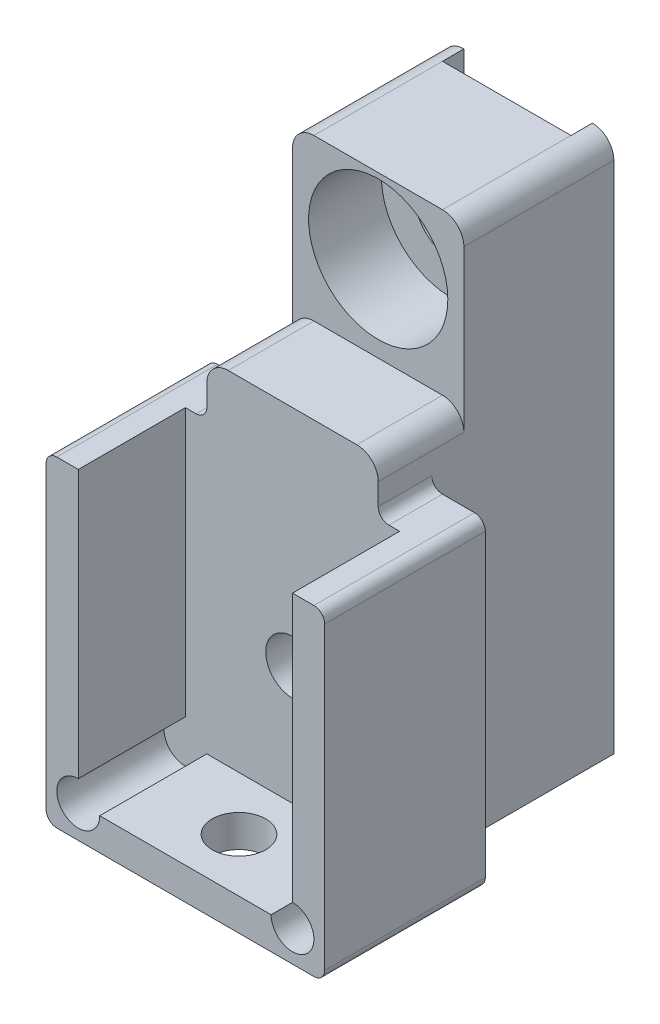
from build123d import *

# Parameters (mm, degrees)
SKETCH1_W                                           = 13
SKETCH1_H                                           = 25
BOSS_EXTRUDE1_DEPTH                                 = 10
CUT_EXTRUDE1_DEPTH                                  = 18.277152543
CUT_EXTRUDE1_DEPTH_BACK                             = 18.277152543
SKETCH2_W                                           = 2.5
SKETCH2_H                                           = 10
FILLET1_R                                           = 0.5
FILLET2_R                                           = 1
SKETCH8_W                                           = 6
SKETCH8_H                                           = 32.589216013
CUT_EXTRUDE4_DEPTH                                  = 1
SKETCH21_W                                          = 10
SKETCH21_H                                          = 30.602707306
CUT_EXTRUDE11_DEPTH                                 = 1
SKETCH25_W                                          = 13.801043237
SKETCH25_H                                          = 15.676526687
CUT_EXTRUDE13_DEPTH                                 = 2
FILLET3_R                                           = 1
CBORE_FOR_M3_HEX_SOCKET_HEAD_CAP_SCREW2_D           = 3.4
CBORE_FOR_M3_HEX_SOCKET_HEAD_CAP_SCREW2_CBORE_D     = 6.5
CBORE_FOR_M3_HEX_SOCKET_HEAD_CAP_SCREW2_CBORE_DEPTH = 5.4
BOSS_EXTRUDE4_START                                 = 6
BOSS_EXTRUDE4_DEPTH                                 = 6
CUT_EXTRUDE15_REACH                                 = 26.109
SKETCH33_W                                          = 10.378798484
SKETCH33_H                                          = 20
SKETCH34_W                                          = 9.92103125
SKETCH34_H                                          = 19.736261401
CUT_EXTRUDE16_DEPTH                                 = 2.5
BOSS_EXTRUDE5_START                                 = 2
BOSS_EXTRUDE5_DEPTH                                 = 2
M3_TAPPED_HOLE1_D                                   = 2.5
M3_TAPPED_HOLE1_DEPTH                               = 7.5
M3_TAPPED_HOLE1_TIP                                 = 0.751075774
M3_TAPPED_HOLE2_D                                   = 2.5
M3_TAPPED_HOLE2_DEPTH                               = 7.5
M3_TAPPED_HOLE2_TIP                                 = 0.751075774
SKETCH41_R                                          = 1
CUT_EXTRUDE17_DEPTH                                 = 5


with BuildPart() as part:
    # Sketch1 → Boss-Extrude1 (new body)
    with BuildSketch(Plane.XY):
        Rectangle(SKETCH1_W, SKETCH1_H)
    extrude(amount=BOSS_EXTRUDE1_DEPTH)

    # Sketch2 → Cut-Extrude1 (cut, two sides: drawn at the far end of the back side and taken through both)
    with BuildSketch(Plane.XY.offset(10).offset(-CUT_EXTRUDE1_DEPTH_BACK)):
        with Locations((-5.25, 7.5)):
            Rectangle(SKETCH2_W, SKETCH2_H)
        with Locations((5.25, 7.5)):
            Rectangle(SKETCH2_W, SKETCH2_H)
    extrude(amount=CUT_EXTRUDE1_DEPTH + CUT_EXTRUDE1_DEPTH_BACK, mode=Mode.SUBTRACT)

    # Fillet1
    fillet1_edges = [part.edges().sort_by_distance(p)[0] for p in [
        (-6.5, 2.5, 5),
        (-4, 2.5, 5),
        (6.5, 2.5, 5),
        (4, 2.5, 5),
        (6.5, -12.5, 5),
        (-6.5, -12.5, 5),
    ]]
    fillet(fillet1_edges, radius=FILLET1_R)

    # Fillet2
    fillet2_edges = [part.edges().sort_by_distance(p)[0] for p in [
        (-4, 12.5, 5),
        (4, 12.5, 5),
    ]]
    fillet(fillet2_edges, radius=FILLET2_R)

    # Sketch8 → Cut-Extrude4 (cut)
    with BuildSketch(Plane(origin=(0, 0, 0), x_dir=(-1, 0, 0), z_dir=(0, 0, -1))):
        with Locations((0, -3.794608007)):
            Rectangle(SKETCH8_W, SKETCH8_H)
    extrude(amount=-CUT_EXTRUDE4_DEPTH, mode=Mode.SUBTRACT)

    # Sketch21 → Cut-Extrude11 (cut)
    with BuildSketch(Plane.XY.offset(10)):
        with Locations((0, 4.301353653)):
            Rectangle(SKETCH21_W, SKETCH21_H)
    extrude(amount=-CUT_EXTRUDE11_DEPTH, mode=Mode.SUBTRACT)

    # Sketch25 → Cut-Extrude13 (cut)
    with BuildSketch(Plane.XY.offset(9)):
        with Locations((-1.252110778, 12.838263344)):
            Rectangle(SKETCH25_W, SKETCH25_H)
    extrude(amount=-CUT_EXTRUDE13_DEPTH, mode=Mode.SUBTRACT)

    # Fillet3
    fillet3_edges = [part.edges().sort_by_distance(p)[0] for p in [
        (4, 5, 8),
        (-4, 5, 8),
    ]]
    fillet(fillet3_edges, radius=FILLET3_R)

    # CBORE for M3 Hex Socket Head Cap Screw2 (through all)
    with Locations(Plane.XY.offset(9)):
        with Locations((0, 9)):
            CounterBoreHole(CBORE_FOR_M3_HEX_SOCKET_HEAD_CAP_SCREW2_D / 2, CBORE_FOR_M3_HEX_SOCKET_HEAD_CAP_SCREW2_CBORE_D / 2, CBORE_FOR_M3_HEX_SOCKET_HEAD_CAP_SCREW2_CBORE_DEPTH)

    # Sketch31 → Boss-Extrude4 (add)
    with BuildSketch(Plane.XY.offset(10).offset(BOSS_EXTRUDE4_START)):
        with BuildLine():
            Line((-5, -11), (-5, 2.5))
            Line((-5, 2.5), (-6, 2.5))
            ThreePointArc((-6, 2.5), (-6.353553391, 2.353553391), (-6.5, 2))
            Line((-6.5, 2), (-6.5, -12))
            ThreePointArc((-6.5, -12), (-6.353553391, -12.353553391), (-6, -12.5))
            Line((-6, -12.5), (6, -12.5))
            ThreePointArc((6, -12.5), (6.353553391, -12.353553391), (6.5, -12))
            Line((6.5, -12), (6.5, 2))
            ThreePointArc((6.5, 2), (6.353553391, 2.353553391), (6, 2.5))
            Line((6, 2.5), (5, 2.5))
            Line((5, 2.5), (5, -11))
            Line((5, -11), (-5, -11))
        make_face()
    extrude(amount=-BOSS_EXTRUDE4_DEPTH)

    # Cut-Extrude15: up to this face of the body (flat: up to its plane)
    cut_extrude15_end = Plane(part.part.faces().sort_by_distance((-4, 7.12804878, 3.646341463))[0])
    # Sketch33 → Cut-Extrude15 (cut, up to the picked face)
    with BuildSketch(Plane.ZY.offset(6.5), mode=Mode.PRIVATE) as cut_extrude15_sk1:
        with Locations((3.310600758, -6.5)):
            Rectangle(SKETCH33_W, SKETCH33_H)
    cut_extrude15_tool1 = split(extrude(cut_extrude15_sk1.sketch, amount=-CUT_EXTRUDE15_REACH, mode=Mode.PRIVATE), bisect_by=cut_extrude15_end, keep=Keep.BOTH, mode=Mode.PRIVATE)
    add(cut_extrude15_tool1.solids().sort_by(Axis((-6.5, -6.5, 3.310601), (1, 0, 0)))[0], mode=Mode.SUBTRACT)

    # Sketch34 → Cut-Extrude16 (cut)
    with BuildSketch(Plane(origin=(6.5, 0, 0), x_dir=(0, 0, -1), z_dir=(1, 0, 0))):
        with Locations((-3.539484375, -6.368130701)):
            Rectangle(SKETCH34_W, SKETCH34_H)
    extrude(amount=-CUT_EXTRUDE16_DEPTH, mode=Mode.SUBTRACT)

    # Sketch36 → Boss-Extrude5 (add)
    with BuildSketch(Plane.XY.offset(9).offset(BOSS_EXTRUDE5_START)):
        with BuildLine():
            Line((-5, 2.5), (-5, -11))
            Line((-5, -11), (5, -11))
            Line((5, -11), (5, 2.5))
            Line((5, 2.5), (4.5, 2.5))
            ThreePointArc((4.5, 2.5), (4.146446609, 2.646446609), (4, 3))
            Line((4, 3), (4, 4))
            ThreePointArc((4, 4), (3.707106781, 4.707106781), (3, 5))
            Line((3, 5), (-3, 5))
            ThreePointArc((-3, 5), (-3.707106781, 4.707106781), (-4, 4))
            Line((-4, 4), (-4, 3))
            ThreePointArc((-4, 3), (-4.146446609, 2.646446609), (-4.5, 2.5))
            Line((-4.5, 2.5), (-5, 2.5))
        make_face()
    extrude(amount=-BOSS_EXTRUDE5_DEPTH)

    # M3 Tapped Hole1
    with Locations(Plane.XY.offset(11)):
        with Locations((0, -5.5)):
            Hole(M3_TAPPED_HOLE1_D / 2, depth=M3_TAPPED_HOLE1_DEPTH)
            with Locations((0, 0, -(M3_TAPPED_HOLE1_DEPTH + M3_TAPPED_HOLE1_TIP / 2))):  # 118° drill point
                Cone(0, M3_TAPPED_HOLE1_D / 2, M3_TAPPED_HOLE1_TIP, mode=Mode.SUBTRACT)

    # M3 Tapped Hole2
    with Locations(Plane(origin=(0, -12.5, 0), x_dir=(-1, 0, 0), z_dir=(0, -1, 0))):
        with Locations((0, -13.5)):
            Hole(M3_TAPPED_HOLE2_D / 2, depth=M3_TAPPED_HOLE2_DEPTH)
            with Locations((0, 0, -(M3_TAPPED_HOLE2_DEPTH + M3_TAPPED_HOLE2_TIP / 2))):  # 118° drill point
                Cone(0, M3_TAPPED_HOLE2_D / 2, M3_TAPPED_HOLE2_TIP, mode=Mode.SUBTRACT)

    # Sketch41 → Cut-Extrude17 (cut)
    with BuildSketch(Plane.XY.offset(16)):
        with Locations((-5, -11)):
            Circle(SKETCH41_R)
        with Locations((5, -11)):
            Circle(SKETCH41_R)
    extrude(amount=-CUT_EXTRUDE17_DEPTH, mode=Mode.SUBTRACT)


solid = part.part
